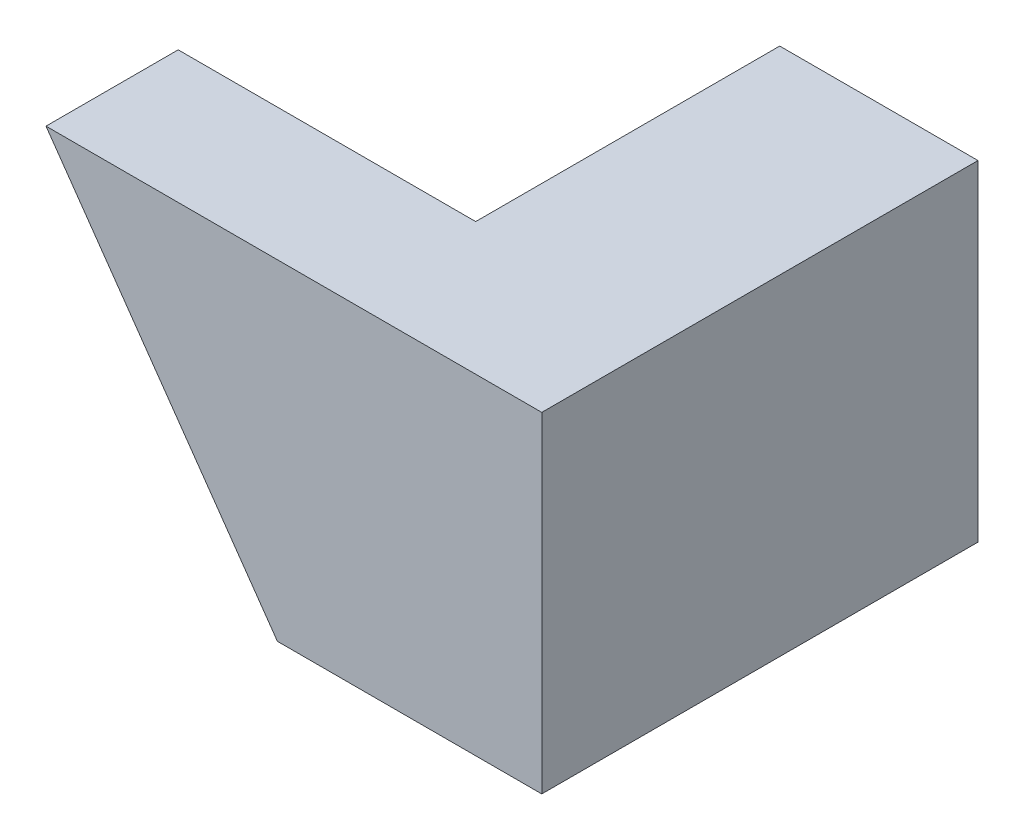
from build123d import *

# Parameters (mm, degrees)
BOSS_EXTRUDE1_DEPTH = 1
SKETCH2_W           = 1.5
SKETCH2_H           = 2.5
BOSS_EXTRUDE2_DEPTH = 3.3


with BuildPart() as part:
    # Sketch1 → Boss-Extrude1 (new body)
    with BuildSketch(Plane.XY):
        Polygon((0, 0), (-1.750518846, 2.5), (2, 2.5), (2, 0), align=None)
    extrude(amount=BOSS_EXTRUDE1_DEPTH)

    # Sketch2 → Boss-Extrude2 (add)
    with BuildSketch(Plane.XY.offset(1)):
        with Locations((1.25, 1.25)):
            Rectangle(SKETCH2_W, SKETCH2_H)
    extrude(amount=-BOSS_EXTRUDE2_DEPTH)


solid = part.part
